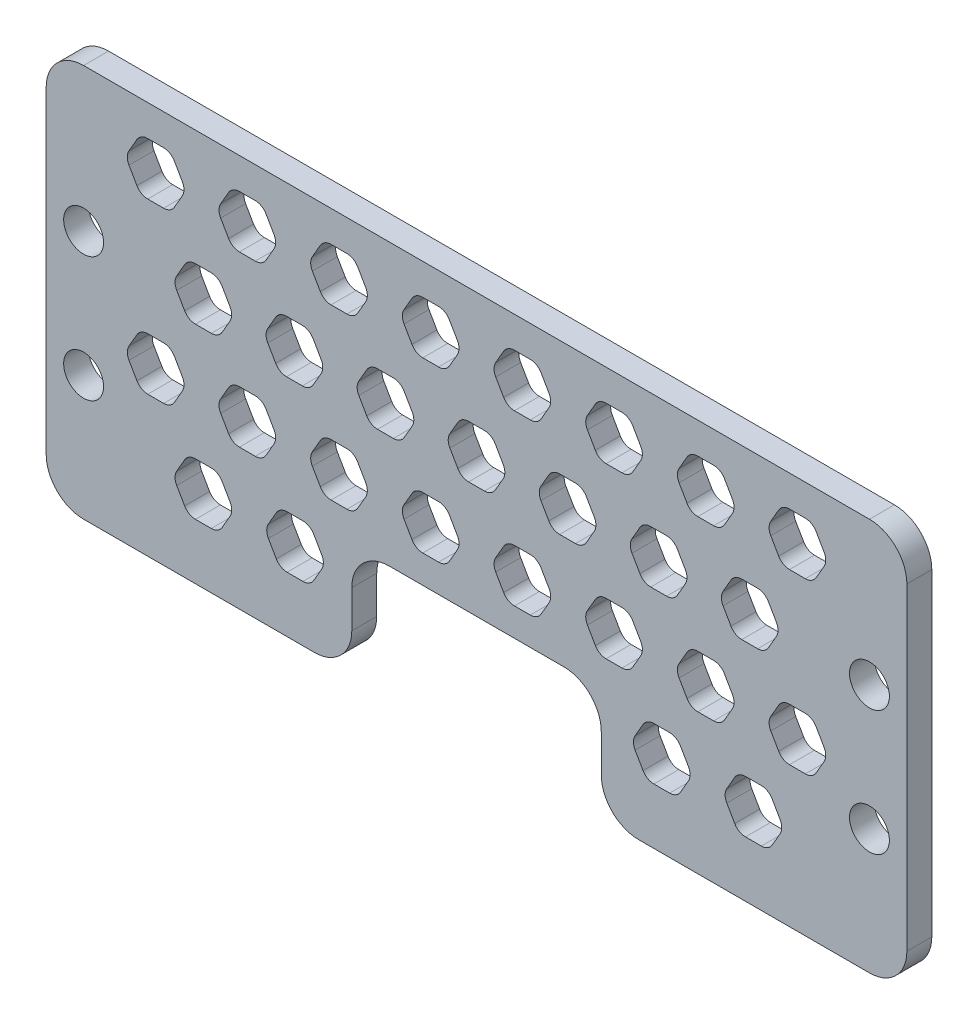
SolidWorks part; units mm, degrees
material "Thornel Mat VMA"
ref_plane "Front Plane" through (0, 0, 0) normal (0, 0, 1) x (1, 0, 0)
ref_plane "Top Plane" through (0, 0, 0) normal (0, 1, 0) x (1, 0, 0)
ref_plane "Right Plane" through (0, 0, 0) normal (1, 0, 0) x (0, 0, -1)
sketch "Sketch1" plane through (0, 0, 0) normal (0, 0, 1) x (1, 0, 0)
  line L0 (0, 15.75) -> (0, -6.75) construction
  line L1 (-34.5, 15.75) -> (34.5, 15.75)
  line L2 (-34.5, 15.75) -> (-34.5, -15.75)
  line L3 (-34.5, -15.75) -> (-10, -15.75)
  line L4 (34.5, 15.75) -> (34.5, -15.75)
  line L5 (-34.5, 15.75) -> (34.5, -15.75) construction
  line L6 (-34.5, -15.75) -> (34.5, 15.75) construction
  line L7 (-31.5, 4.25) -> (-31.5, -5.75) construction
  line L8 (31.5, 4.25) -> (31.5, -5.75) construction
  line L9 (-10, -15.75) -> (-10, -6.75)
  line L10 (10, -15.75) -> (10, -6.75)
  line L11 (-10, -6.75) -> (10, -6.75)
  line L12 (10, -15.75) -> (34.5, -15.75)
  circle A0 centre (-31.5, 4.25) radius 1.6
  circle A1 centre (-31.5, -5.75) radius 1.6
  circle A2 centre (31.5, -5.75) radius 1.6
  circle A3 centre (31.5, 4.25) radius 1.6
  point P0 (0, 0)
  dimension "D1" = 69
  dimension "D3" = 3.2
  dimension "D2" = 31.5
  dimension "D4" = 10
  dimension "D5" = 3
  dimension "D6" = 20
  dimension "D7" = 9
  dimension "D8" = 11.5
extrude "Boss-Extrude1" add sketch "Sketch1" along normal blind 2
sketch "Sketch2" plane through (0, 0, 2) normal (0, 0, 1) x (1, 0, 0)
  line L0 (-28.149, 11.15) -> (-26.9365, 13.25)
  line L1 (-26.9365, 13.25) -> (-24.5117, 13.25)
  line L2 (-24.5117, 13.25) -> (-23.2992, 11.15)
  line L3 (-23.2992, 11.15) -> (-24.5117, 9.05)
  line L4 (-24.5117, 9.05) -> (-26.9365, 9.05)
  line L5 (-26.9365, 9.05) -> (-28.149, 11.15)
  line L6 (-19.5868, 9.05) -> (-20.7992, 11.15)
  line L7 (-20.7992, 11.15) -> (-19.5868, 13.25)
  line L8 (-19.5868, 13.25) -> (-17.1619, 13.25)
  line L9 (-17.1619, 13.25) -> (-15.9495, 11.15)
  line L10 (-15.9495, 11.15) -> (-17.1619, 9.05)
  line L11 (-17.1619, 9.05) -> (-19.5868, 9.05)
  line L12 (-12.237, 9.05) -> (-13.4495, 11.15)
  line L13 (-13.4495, 11.15) -> (-12.237, 13.25)
  line L14 (-12.237, 13.25) -> (-9.8122, 13.25)
  line L15 (-9.8122, 13.25) -> (-8.5997, 11.15)
  line L16 (-8.5997, 11.15) -> (-9.8122, 9.05)
  line L17 (-9.8122, 9.05) -> (-12.237, 9.05)
  line L18 (-4.8873, 9.05) -> (-6.0997, 11.15)
  line L19 (-6.0997, 11.15) -> (-4.8873, 13.25)
  line L20 (-4.8873, 13.25) -> (-2.4624, 13.25)
  line L21 (-2.4624, 13.25) -> (-1.25, 11.15)
  line L22 (-1.25, 11.15) -> (-2.4624, 9.05)
  line L23 (-2.4624, 9.05) -> (-4.8873, 9.05)
  line L24 (2.4624, 9.05) -> (1.25, 11.15)
  line L25 (1.25, 11.15) -> (2.4624, 13.25)
  line L26 (2.4624, 13.25) -> (4.8873, 13.25)
  line L27 (4.8873, 13.25) -> (6.0997, 11.15)
  line L28 (6.0997, 11.15) -> (4.8873, 9.05)
  line L29 (4.8873, 9.05) -> (2.4624, 9.05)
  line L30 (9.8122, 9.05) -> (8.5997, 11.15)
  line L31 (8.5997, 11.15) -> (9.8122, 13.25)
  line L32 (9.8122, 13.25) -> (12.237, 13.25)
  line L33 (12.237, 13.25) -> (13.4495, 11.15)
  line L34 (13.4495, 11.15) -> (12.237, 9.05)
  line L35 (12.237, 9.05) -> (9.8122, 9.05)
  line L36 (17.1619, 9.05) -> (15.9495, 11.15)
  line L37 (15.9495, 11.15) -> (17.1619, 13.25)
  line L38 (17.1619, 13.25) -> (19.5868, 13.25)
  line L39 (19.5868, 13.25) -> (20.7992, 11.15)
  line L40 (20.7992, 11.15) -> (19.5868, 9.05)
  line L41 (19.5868, 9.05) -> (17.1619, 9.05)
  line L42 (24.5117, 9.05) -> (23.2992, 11.15)
  line L43 (23.2992, 11.15) -> (24.5117, 13.25)
  line L44 (24.5117, 13.25) -> (26.9365, 13.25)
  line L45 (26.9365, 13.25) -> (28.149, 11.15)
  line L46 (28.149, 11.15) -> (26.9365, 9.05)
  line L47 (26.9365, 9.05) -> (24.5117, 9.05)
  line L48 (0, 15.75) -> (0, -6.75) construction
  line L49 (34.5, 15.75) -> (-34.5, 15.75) construction
  line L50 (-10, -6.75) -> (10, -6.75) construction
  line L51 (-24.3241, 4.3749) -> (-23.1117, 6.4749)
  line L52 (-23.1117, 6.4749) -> (-20.6868, 6.4749)
  line L53 (-20.6868, 6.4749) -> (-19.4744, 4.3749)
  line L54 (-19.4744, 4.3749) -> (-20.6868, 2.2749)
  line L55 (-20.6868, 2.2749) -> (-23.1117, 2.2749)
  line L56 (-23.1117, 2.2749) -> (-24.3241, 4.3749)
  line L57 (-15.8119, 2.2749) -> (-17.0244, 4.3749)
  line L58 (-17.0244, 4.3749) -> (-15.8119, 6.4749)
  line L59 (-15.8119, 6.4749) -> (-13.387, 6.4749)
  line L60 (-13.387, 6.4749) -> (-12.1746, 4.3749)
  line L61 (-12.1746, 4.3749) -> (-13.387, 2.2749)
  line L62 (-13.387, 2.2749) -> (-15.8119, 2.2749)
  line L63 (-8.5122, 2.2749) -> (-9.7246, 4.3749)
  line L64 (-9.7246, 4.3749) -> (-8.5122, 6.4749)
  line L65 (-8.5122, 6.4749) -> (-6.0873, 6.4749)
  line L66 (-6.0873, 6.4749) -> (-4.8749, 4.3749)
  line L67 (-4.8749, 4.3749) -> (-6.0873, 2.2749)
  line L68 (-6.0873, 2.2749) -> (-8.5122, 2.2749)
  line L69 (-1.2124, 2.2749) -> (-2.4249, 4.3749)
  line L70 (-2.4249, 4.3749) -> (-1.2124, 6.4749)
  line L71 (-1.2124, 6.4749) -> (1.2124, 6.4749)
  line L72 (1.2124, 6.4749) -> (2.4249, 4.3749)
  line L73 (2.4249, 4.3749) -> (1.2124, 2.2749)
  line L74 (1.2124, 2.2749) -> (-1.2124, 2.2749)
  line L75 (6.0873, 2.2749) -> (4.8749, 4.3749)
  line L76 (4.8749, 4.3749) -> (6.0873, 6.4749)
  line L77 (6.0873, 6.4749) -> (8.5122, 6.4749)
  line L78 (8.5122, 6.4749) -> (9.7246, 4.3749)
  line L79 (9.7246, 4.3749) -> (8.5122, 2.2749)
  line L80 (8.5122, 2.2749) -> (6.0873, 2.2749)
  line L81 (13.387, 2.2749) -> (12.1746, 4.3749)
  line L82 (12.1746, 4.3749) -> (13.387, 6.4749)
  line L83 (13.387, 6.4749) -> (15.8119, 6.4749)
  line L84 (15.8119, 6.4749) -> (17.0244, 4.3749)
  line L85 (17.0244, 4.3749) -> (15.8119, 2.2749)
  line L86 (15.8119, 2.2749) -> (13.387, 2.2749)
  line L87 (20.6868, 2.2749) -> (19.4744, 4.3749)
  line L88 (19.4744, 4.3749) -> (20.6868, 6.4749)
  line L89 (20.6868, 6.4749) -> (23.1117, 6.4749)
  line L90 (23.1117, 6.4749) -> (24.3241, 4.3749)
  line L91 (24.3241, 4.3749) -> (23.1117, 2.2749)
  line L92 (23.1117, 2.2749) -> (20.6868, 2.2749)
  line L93 (-24.3241, 4.3749) -> (-19.4744, 4.3749) construction
  line L94 (-26.9365, -4.5003) -> (-28.149, -2.4003)
  line L95 (-28.149, -2.4003) -> (-26.9365, -0.3003)
  line L96 (-26.9365, -0.3003) -> (-24.5117, -0.3003)
  line L97 (-24.5117, -0.3003) -> (-23.2992, -2.4003)
  line L98 (-23.2992, -2.4003) -> (-24.5117, -4.5003)
  line L99 (-24.5117, -4.5003) -> (-26.9365, -4.5003)
  line L100 (-19.5868, -4.5003) -> (-20.7992, -2.4003)
  line L101 (-20.7992, -2.4003) -> (-19.5868, -0.3003)
  line L102 (-19.5868, -0.3003) -> (-17.1619, -0.3003)
  line L103 (-17.1619, -0.3003) -> (-15.9495, -2.4003)
  line L104 (-15.9495, -2.4003) -> (-17.1619, -4.5003)
  line L105 (-17.1619, -4.5003) -> (-19.5868, -4.5003)
  line L106 (-12.237, -4.5003) -> (-13.4495, -2.4003)
  line L107 (-13.4495, -2.4003) -> (-12.237, -0.3003)
  line L108 (-12.237, -0.3003) -> (-9.8122, -0.3003)
  line L109 (-9.8122, -0.3003) -> (-8.5997, -2.4003)
  line L110 (-8.5997, -2.4003) -> (-9.8122, -4.5003)
  line L111 (-9.8122, -4.5003) -> (-12.237, -4.5003)
  line L112 (-4.8873, -4.5003) -> (-6.0997, -2.4003)
  line L113 (-6.0997, -2.4003) -> (-4.8873, -0.3003)
  line L114 (-4.8873, -0.3003) -> (-2.4624, -0.3003)
  line L115 (-2.4624, -0.3003) -> (-1.25, -2.4003)
  line L116 (-1.25, -2.4003) -> (-2.4624, -4.5003)
  line L117 (-2.4624, -4.5003) -> (-4.8873, -4.5003)
  line L118 (2.4624, -4.5003) -> (1.25, -2.4003)
  line L119 (1.25, -2.4003) -> (2.4624, -0.3003)
  line L120 (2.4624, -0.3003) -> (4.8873, -0.3003)
  line L121 (4.8873, -0.3003) -> (6.0997, -2.4003)
  line L122 (6.0997, -2.4003) -> (4.8873, -4.5003)
  line L123 (4.8873, -4.5003) -> (2.4624, -4.5003)
  line L124 (9.8122, -4.5003) -> (8.5997, -2.4003)
  line L125 (8.5997, -2.4003) -> (9.8122, -0.3003)
  line L126 (9.8122, -0.3003) -> (12.237, -0.3003)
  line L127 (12.237, -0.3003) -> (13.4495, -2.4003)
  line L128 (13.4495, -2.4003) -> (12.237, -4.5003)
  line L129 (12.237, -4.5003) -> (9.8122, -4.5003)
  line L130 (17.1619, -4.5003) -> (15.9495, -2.4003)
  line L131 (15.9495, -2.4003) -> (17.1619, -0.3003)
  line L132 (17.1619, -0.3003) -> (19.5868, -0.3003)
  line L133 (19.5868, -0.3003) -> (20.7992, -2.4003)
  line L134 (20.7992, -2.4003) -> (19.5868, -4.5003)
  line L135 (19.5868, -4.5003) -> (17.1619, -4.5003)
  line L136 (24.5117, -4.5003) -> (23.2992, -2.4003)
  line L137 (23.2992, -2.4003) -> (24.5117, -0.3003)
  line L138 (24.5117, -0.3003) -> (26.9365, -0.3003)
  line L139 (26.9365, -0.3003) -> (28.149, -2.4003)
  line L140 (28.149, -2.4003) -> (26.9365, -4.5003)
  line L141 (26.9365, -4.5003) -> (24.5117, -4.5003)
  line L142 (-24.3241, -9.1754) -> (-23.1117, -7.0754)
  line L143 (-23.1117, -7.0754) -> (-20.6868, -7.0754)
  line L144 (-20.6868, -7.0754) -> (-19.4744, -9.1754)
  line L145 (-19.4744, -9.1754) -> (-20.6868, -11.2754)
  line L146 (-20.6868, -11.2754) -> (-23.1117, -11.2754)
  line L147 (-23.1117, -11.2754) -> (-24.3241, -9.1754)
  line L166 (-15.7619, -11.2754) -> (-16.9744, -9.1754)
  line L167 (-16.9744, -9.1754) -> (-15.7619, -7.0754)
  line L168 (-15.7619, -7.0754) -> (-13.337, -7.0754)
  line L169 (-13.337, -7.0754) -> (-12.1246, -9.1754)
  line L170 (-12.1246, -9.1754) -> (-13.337, -11.2754)
  line L171 (-13.337, -11.2754) -> (-15.7619, -11.2754)
  line L172 (-8.4122, -11.2754) -> (-9.6246, -9.1754) construction
  line L173 (-9.6246, -9.1754) -> (-8.4122, -7.0754) construction
  line L174 (-8.4122, -7.0754) -> (-5.9873, -7.0754) construction
  line L175 (-5.9873, -7.0754) -> (-4.7749, -9.1754) construction
  line L176 (-4.7749, -9.1754) -> (-5.9873, -11.2754) construction
  line L177 (-5.9873, -11.2754) -> (-8.4122, -11.2754) construction
  line L178 (-1.0624, -11.2754) -> (-2.2749, -9.1754) construction
  line L179 (-2.2749, -9.1754) -> (-1.0624, -7.0754) construction
  line L180 (-1.0624, -7.0754) -> (1.3624, -7.0754) construction
  line L181 (1.3624, -7.0754) -> (2.5749, -9.1754) construction
  line L182 (2.5749, -9.1754) -> (1.3624, -11.2754) construction
  line L183 (1.3624, -11.2754) -> (-1.0624, -11.2754) construction
  line L184 (6.2873, -11.2754) -> (5.0749, -9.1754) construction
  line L185 (5.0749, -9.1754) -> (6.2873, -7.0754) construction
  line L186 (6.2873, -7.0754) -> (8.7122, -7.0754) construction
  line L187 (8.7122, -7.0754) -> (9.9246, -9.1754) construction
  line L188 (9.9246, -9.1754) -> (8.7122, -11.2754) construction
  line L189 (8.7122, -11.2754) -> (6.2873, -11.2754) construction
  line L190 (13.637, -11.2754) -> (12.4246, -9.1754)
  line L191 (12.4246, -9.1754) -> (13.637, -7.0754)
  line L192 (13.637, -7.0754) -> (16.0619, -7.0754)
  line L193 (16.0619, -7.0754) -> (17.2744, -9.1754)
  line L194 (17.2744, -9.1754) -> (16.0619, -11.2754)
  line L195 (16.0619, -11.2754) -> (13.637, -11.2754)
  line L196 (20.9868, -11.2754) -> (19.7744, -9.1754)
  line L197 (19.7744, -9.1754) -> (20.9868, -7.0754)
  line L198 (20.9868, -7.0754) -> (23.4117, -7.0754)
  line L199 (23.4117, -7.0754) -> (24.6241, -9.1754)
  line L200 (24.6241, -9.1754) -> (23.4117, -11.2754)
  line L201 (23.4117, -11.2754) -> (20.9868, -11.2754)
  circle A0 centre (-25.7241, 11.15) radius 2.4249 construction
  circle A1 centre (-21.8992, 4.3749) radius 2.4249 construction
  circle A2 centre (-21.8992, -9.1754) radius 2.4249 construction
  dimension "D1" = 4.2
  dimension "D5" = 1.4
  dimension "D10" = 2.5
  dimension "D3" = 2.5
  dimension "D4" = 2.5
  dimension "D6" = 2.5
  dimension "D8" = 2
  dimension "D9" = 2.5
  dimension "D11" = 7
  dimension "D12" = 2.5
  dimension "D2" = 8
  dimension "D7" = 7
extrude "Cut-Extrude1" cut sketch "Sketch2" against normal through all
fillet "R1 cutout fillet" radius 1 119 edges at (-28.149, 11.15, 1) (-26.9365, 13.25, 1) (-24.5117, 13.25, 1) (-24.5117, 9.05, 1) (-26.9365, 9.05, 1) (-15.7619, -7.0754, 1) (-13.337, -7.0754, 1) (-12.1246, -9.1754, 1) (-13.337, -11.2754, 1) (-15.7619, -11.2754, 1) (-24.3241, -9.1754, 1) (-20.6868, -7.0754, 1) (-19.4744, -9.1754, 1) (24.5117, -0.3003, 1) (26.9365, -0.3003, 1) (26.9365, -4.5003, 1) (24.5117, -4.5003, 1) (23.2992, -2.4003, 1) (17.1619, -0.3003, 1) (19.5868, -0.3003, 1) (20.7992, -2.4003, 1) (19.5868, -4.5003, 1) (17.1619, -4.5003, 1) (15.9495, -2.4003, 1) (12.237, -0.3003, 1) (13.4495, -2.4003, 1) (9.8122, -4.5003, 1) (8.5997, -2.4003, 1) (4.8873, -0.3003, 1) (6.0997, -2.4003, 1) (4.8873, -4.5003, 1) (2.4624, -4.5003, 1) (1.25, -2.4003, 1) (-4.8873, -0.3003, 1) (-1.25, -2.4003, 1) (-2.4624, -4.5003, 1) (-6.0997, -2.4003, 1) (-9.8122, -0.3003, 1) (-9.8122, -4.5003, 1) (-13.4495, -2.4003, 1) (13.637, -7.0754, 1) (17.2744, -9.1754, 1) (16.0619, -11.2754, 1) (13.637, -11.2754, 1) (12.4246, -9.1754, 1) (20.9868, -7.0754, 1) (23.4117, -7.0754, 1) (23.4117, -11.2754, 1) (20.9868, -11.2754, 1) (19.7744, -9.1754, 1) (9.8122, 13.25, 1) (12.237, 13.25, 1) (13.4495, 11.15, 1) (9.8122, 9.05, 1) (8.5997, 11.15, 1) (19.5868, 13.25, 1) (20.7992, 11.15, 1) (19.5868, 9.05, 1) (15.9495, 11.15, 1) (24.5117, 13.25, 1) (26.9365, 13.25, 1) (28.149, 11.15, 1) (24.5117, 9.05, 1) (23.2992, 11.15, 1) (-23.1117, 6.4749, 1) (-19.4744, 4.3749, 1) (-20.6868, 2.2749, 1) (-23.1117, 2.2749, 1) (2.4624, 13.25, 1) (6.0997, 11.15, 1) (4.8873, 9.05, 1) (-2.4624, 13.25, 1) (-1.25, 11.15, 1) (-2.4624, 9.05, 1) (-4.8873, 9.05, 1) (-9.8122, 13.25, 1) (-8.5997, 11.15, 1) (-9.8122, 9.05, 1) (-13.4495, 11.15, 1) (-19.5868, 13.25, 1) (-15.9495, 11.15, 1) (-17.1619, 9.05, 1) (-19.5868, 9.05, 1) (6.0873, 6.4749, 1) (8.5122, 6.4749, 1) (9.7246, 4.3749, 1) (8.5122, 2.2749, 1) (6.0873, 2.2749, 1) (13.387, 6.4749, 1) (17.0244, 4.3749, 1) (15.8119, 2.2749, 1) (13.387, 2.2749, 1) (12.1746, 4.3749, 1) (20.6868, 6.4749, 1) (24.3241, 4.3749, 1) (23.1117, 2.2749, 1) (19.4744, 4.3749, 1) (-19.5868, -0.3003, 1) (-17.1619, -0.3003, 1) (-15.9495, -2.4003, 1) (-17.1619, -4.5003, 1) (-19.5868, -4.5003, 1) (-20.7992, -2.4003, 1) (1.2124, 6.4749, 1) (-1.2124, 2.2749, 1) (-2.4249, 4.3749, 1) (-8.5122, 6.4749, 1) (-6.0873, 6.4749, 1) (-4.8749, 4.3749, 1) (-13.387, 6.4749, 1) (-13.387, 2.2749, 1) (-15.8119, 2.2749, 1) (-17.0244, 4.3749, 1) (-26.9365, -0.3003, 1) (-23.2992, -2.4003, 1) (-24.5117, -4.5003, 1) (-26.9365, -4.5003, 1) (-28.149, -2.4003, 1) (-23.2992, 11.15, 1)
fillet "R3 outer edge fillet" radius 3 8 edges at (10, -15.75, 1) (10, -6.75, 1) (-10, -6.75, 1) (-34.5, -15.75, 1) (-34.5, 15.75, 1) (34.5, 15.75, 1) (34.5, -15.75, 1) (-10, -15.75, 1)
